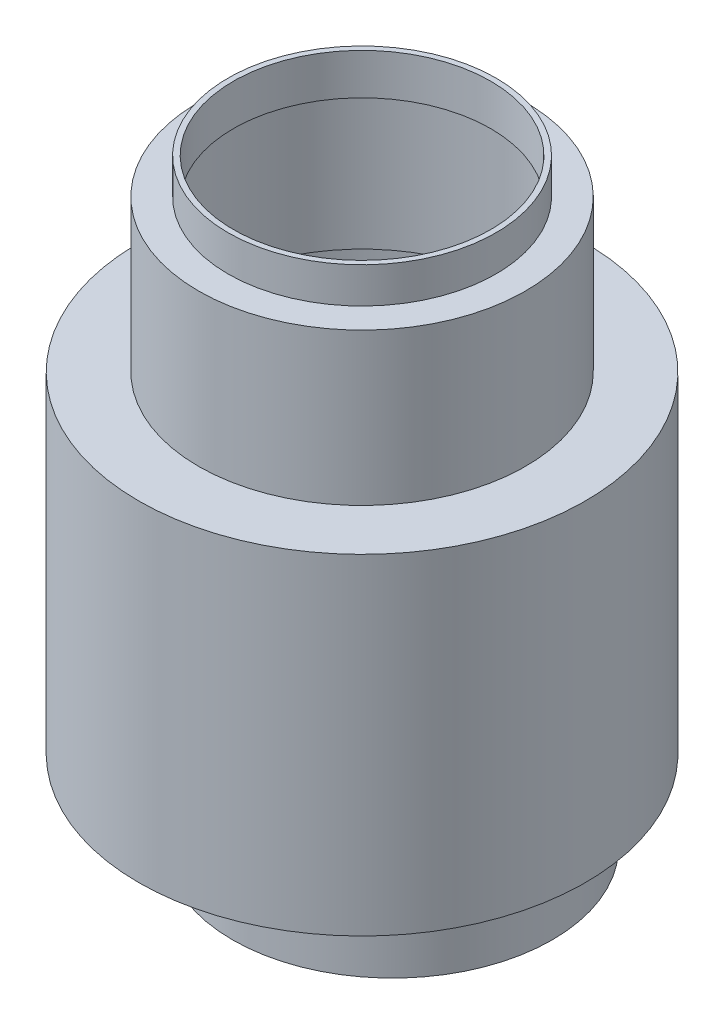
from build123d import *

# Parameters (mm, degrees)
SKETCH2_R           = 89.5
BOSS_EXTRUDE1_DEPTH = 37
SHELL1_T            = -3


with BuildPart() as part:
    # Sketch1 → Revolve1 (revolve)
    with BuildSketch(Plane.XY, mode=Mode.PRIVATE) as revolve1_sk:
        Polygon((0, 0), (125, 0), (125, 185), (91.5, 185), (91.5, 270), (75, 270), (75, 290), (0, 290), align=None)
    revolve(revolve1_sk.sketch.rotate(Axis((0, 290, 0), (0, -1, 0)), 90), axis=Axis((0, 290, 0), (0, -1, 0)))

    # Sketch2 → Boss-Extrude1 (add)
    with BuildSketch(Plane.XZ):
        with Locations(Location((17, 0, 0), (0, 0, 90))):
            Circle(SKETCH2_R)
    extrude(amount=BOSS_EXTRUDE1_DEPTH)

    # Shell1
    shell1_openings = [part.faces().sort_by_distance(p)[0] for p in [
        (17, -37, 0),
        (0, 290, 0),
    ]]
    offset(amount=SHELL1_T, openings=shell1_openings, kind=Kind.INTERSECTION)


solid = part.part
